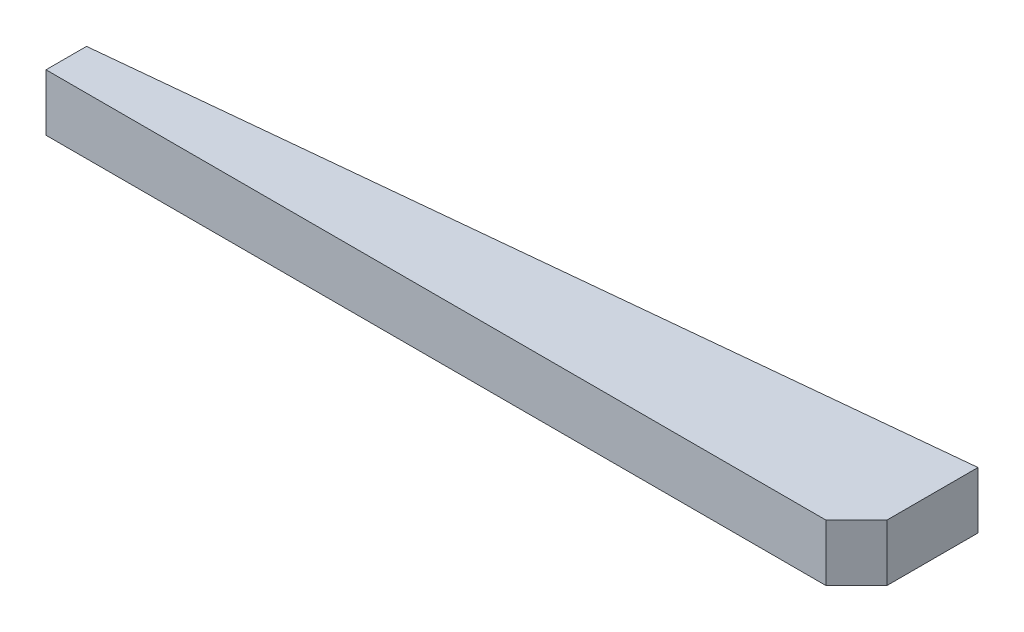
SolidWorks part; units mm, degrees
ref_plane "Front Plane" through (0, 0, 0) normal (0, 0, 1) x (1, 0, 0)
ref_plane "Top Plane" through (0, 0, 0) normal (0, 1, 0) x (1, 0, 0)
ref_plane "Right Plane" through (0, 0, 0) normal (1, 0, 0) x (0, 0, -1)
sketch "Sketch1" plane through (0, 0, 0) normal (0, 1, 0) x (1, 0, 0)
  line L0 (2011.5239, 1584.0079) -> (2396.5239, 1584.0079)
  line L1 (2396.5239, 1584.0079) -> (2411.5239, 1599.0079)
  line L2 (2411.5239, 1599.0079) -> (2411.5239, 1644.0079)
  line L3 (2411.5239, 1644.0079) -> (2011.5239, 1604.0079)
  line L4 (2011.5239, 1604.0079) -> (2011.5239, 1584.0079)
extrude "Boss-Extrude1" add sketch "Sketch1" along normal blind 28
